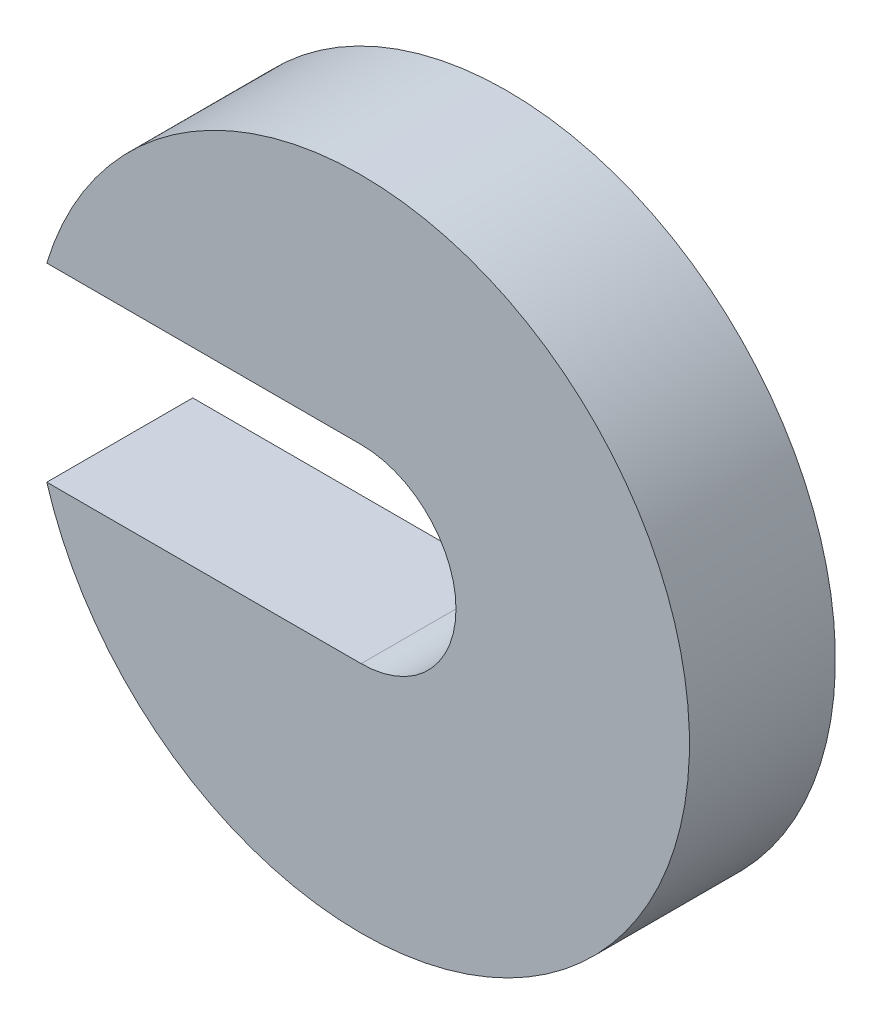
SolidWorks part; units mm, degrees
ref_plane "Front Plane" through (0, 0, 0) normal (0, 0, 1) x (1, 0, 0)
ref_plane "Top Plane" through (0, 0, 0) normal (0, 1, 0) x (1, 0, 0)
ref_plane "Right Plane" through (0, 0, 0) normal (1, 0, 0) x (0, 0, -1)
sketch "Sketch1" plane through (0, 0, 0) normal (0, 0, 1) x (1, 0, 0)
  line L0 (0, 6.5) -> (-21.5407, 6.5)
  line L1 (0, -6.5) -> (-21.5407, -6.5)
  arc A0 (-21.5407, -6.5) -> (-21.5407, 6.5) centre (0, 0) ccw
  arc A1 (0, -6.5) -> (0, 6.5) centre (0, 0) ccw
extrude "Boss-Extrude1" add sketch "Sketch1" along normal blind 10
